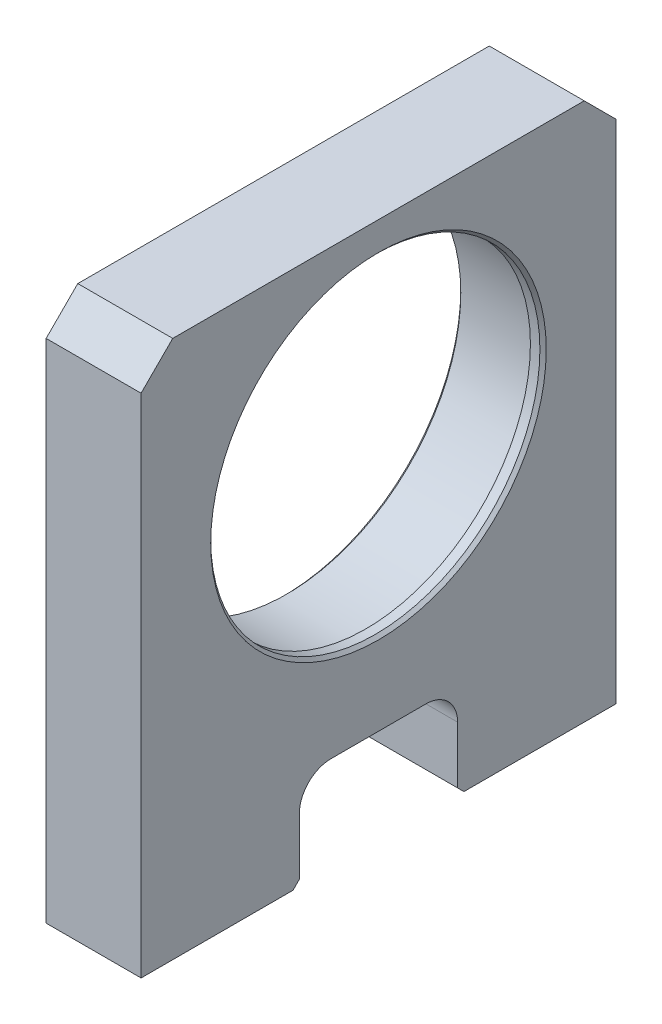
from build123d import *

# Parameters (mm, degrees)
SKETCH1_R             = 27.5
BOSS_EXTRUDE2_DEPTH   = 7.5
M6_TAPPED_HOLE1_D     = 5
M6_TAPPED_HOLE1_DEPTH = 17
M6_TAPPED_HOLE1_TIP   = 1.502151548
BOSS_EXTRUDE3_START   = -2
SKETCH5_R             = 27.5
SKETCH5_R_2           = 26
BOSS_EXTRUDE3_DEPTH   = 2
CHAMFER1_SIZE         = 5
SKETCH4_R             = 2.5
CUT_EXTRUDE1_DEPTH    = 15
CHAMFER2_SIZE         = 1
CHAMFER3_SIZE         = 0.5


with BuildPart() as part:
    # Sketch1 → Boss-Extrude2 (new, symmetric)
    with BuildSketch(Plane(origin=(0, 0, 0), x_dir=(0, 0, -1), z_dir=(1, 0, 0))):
        with BuildLine():
            Line((-37.5, -42.5), (-12.5, -42.5))
            Line((-12.5, -42.5), (-12.5, -32.5))
            ThreePointArc((-12.5, -32.5), (-11.035533906, -28.964466094), (-7.5, -27.5))
            Line((-7.5, -27.5), (7.5, -27.5))
            ThreePointArc((7.5, -27.5), (11.035533906, -28.964466094), (12.5, -32.5))
            Line((12.5, -32.5), (12.5, -42.5))
            Line((12.5, -42.5), (37.5, -42.5))
            Line((37.5, -42.5), (37.5, 42.5))
            Line((37.5, 42.5), (-37.5, 42.5))
            Line((-37.5, 42.5), (-37.5, -42.5))
        make_face()
        with Locations((0, 11.5)):
            Circle(SKETCH1_R, mode=Mode.SUBTRACT)
    extrude(amount=BOSS_EXTRUDE2_DEPTH, both=True)

    # M6 Tapped Hole1
    with Locations(Plane(origin=(0, -42.5, 0), x_dir=(-1, 0, 0), z_dir=(0, -1, 0))):
        with Locations((0, -32.5), (0, 32.5)):
            Hole(M6_TAPPED_HOLE1_D / 2, depth=M6_TAPPED_HOLE1_DEPTH)
            with Locations((0, 0, -(M6_TAPPED_HOLE1_DEPTH + M6_TAPPED_HOLE1_TIP / 2))):  # 118° drill point
                Cone(0, M6_TAPPED_HOLE1_D / 2, M6_TAPPED_HOLE1_TIP, mode=Mode.SUBTRACT)

    # Sketch5 → Boss-Extrude3 (add)
    with BuildSketch(Plane(origin=(7.5, 0, 0), x_dir=(0, 0, -1), z_dir=(1, 0, 0)).offset(BOSS_EXTRUDE3_START)):
        with Locations((0, 11.5)):
            Circle(SKETCH5_R)
        with Locations((0, 11.5)):
            Circle(SKETCH5_R_2, mode=Mode.SUBTRACT)
    extrude(amount=BOSS_EXTRUDE3_DEPTH)

    # Chamfer1
    chamfer1_edges = [part.edges().sort_by_distance(p)[0] for p in [
        (0, 42.5, 37.5),
        (0, 42.5, -37.5),
    ]]
    chamfer(chamfer1_edges, length=CHAMFER1_SIZE)

    # Sketch4 → Cut-Extrude1 (cut)
    with BuildSketch(Plane.XZ.offset(42.5)):
        with Locations(Location((0, -20, 0), (0, 0, 270))):
            Circle(SKETCH4_R)
        with BuildLine():
            Line((2.5, 20.5), (2.5, 19.5))
            ThreePointArc((2.5, 19.5), (0, 17), (-2.5, 19.5))
            Line((-2.5, 19.5), (-2.5, 20.5))
            ThreePointArc((-2.5, 20.5), (0, 23), (2.5, 20.5))
        make_face()
    extrude(amount=-CUT_EXTRUDE1_DEPTH, mode=Mode.SUBTRACT)

    # Chamfer2
    chamfer2_edges = [part.edges().sort_by_distance(p)[0] for p in [
        (0, -42.5, -12.5),
        (0, -42.5, 12.5),
    ]]
    chamfer(chamfer2_edges, length=CHAMFER2_SIZE)

    # Chamfer3
    chamfer3_edges = [part.edges().sort_by_distance(p)[0] for p in [
        (-7.5, 11.5, 27.5),
        (7.5, 11.5, 26),
    ]]
    chamfer(chamfer3_edges, length=CHAMFER3_SIZE)


solid = part.part
